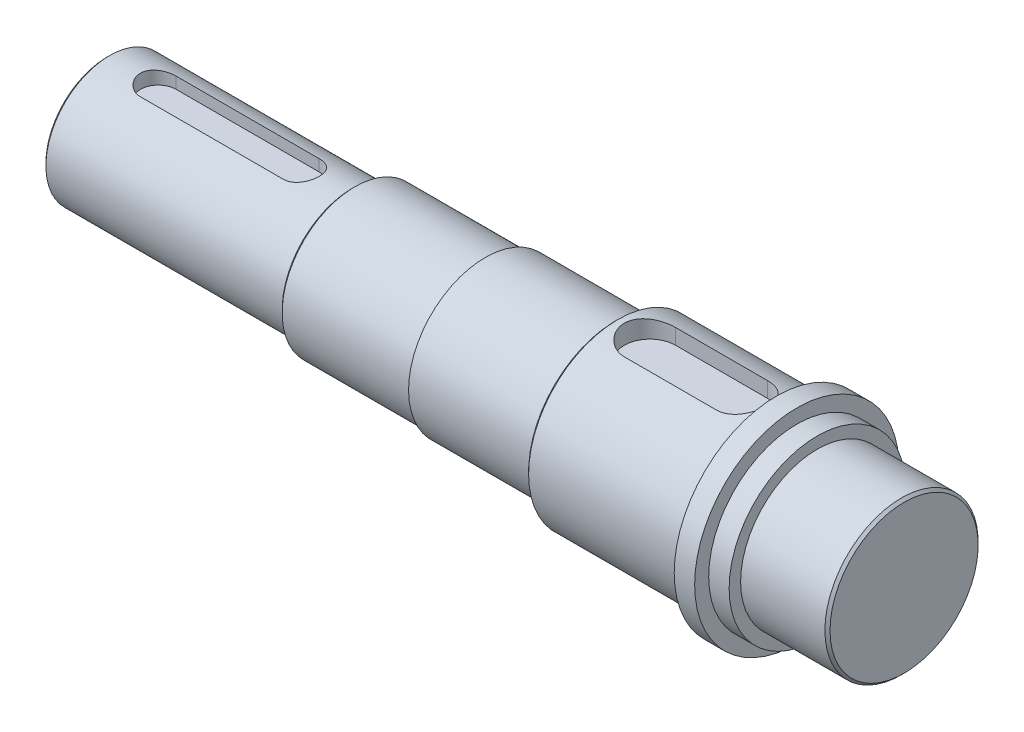
from build123d import *

# Parameters (mm, degrees)
CHAMFER1_SIZE      = 1
CHAMFER2_SIZE      = 1
FILLET1_R          = 0.5
CHAMFER3_SIZE      = 1
CHAMFER4_SIZE      = 1
FILLET2_R          = 0.5
CUT_EXTRUDE1_START = 19.5
CUT_EXTRUDE1_DEPTH = 20
CUT_EXTRUDE2_START = 27.5
CUT_EXTRUDE2_DEPTH = 20


with BuildPart() as part:
    # Sketch1 → Revolve3 (revolve)
    with BuildSketch(Plane.XY, mode=Mode.PRIVATE) as revolve3_sk:
        Polygon((0, 0), (0, 25), (96, 25), (96, 28.5), (148, 28.5), (148, 30), (199, 30), (199, 35), (262, 35), (262, 40), (270, 40), (270, 34.5), (278, 34.5), (278, 30), (312, 30), (312, 0), align=None)
    revolve(revolve3_sk.sketch.rotate(Axis((0, 0, 0), (1, 0, 0)), 90), axis=Axis((0, 0, 0), (1, 0, 0)))

    # Chamfer1
    chamfer1_edges = [part.edges().sort_by_distance(p)[0] for p in [
        (0, 0, -25),
    ]]
    chamfer(chamfer1_edges, length=CHAMFER1_SIZE)

    # Chamfer2
    chamfer2_edges = [part.edges().sort_by_distance(p)[0] for p in [
        (312, 0, -30),
    ]]
    chamfer(chamfer2_edges, length=CHAMFER2_SIZE)

    # Fillet1
    fillet1_edges = [part.edges().sort_by_distance(p)[0] for p in [
        (148, 0, -28.5),
        (96, 0, -25),
    ]]
    fillet(fillet1_edges, radius=FILLET1_R)

    # Chamfer3
    chamfer3_edges = [part.edges().sort_by_distance(p)[0] for p in [
        (199, 0, -35),
    ]]
    chamfer(chamfer3_edges, length=CHAMFER3_SIZE)

    # Chamfer4
    chamfer4_edges = [part.edges().sort_by_distance(p)[0] for p in [
        (96, 0, -28.5),
    ]]
    chamfer(chamfer4_edges, length=CHAMFER4_SIZE)

    # Fillet2
    fillet2_edges = [part.edges().sort_by_distance(p)[0] for p in [
        (199, 0, -30),
    ]]
    fillet(fillet2_edges, radius=FILLET2_R)

    # Sketch2 → Cut-Extrude1 (cut)
    with BuildSketch(Plane(origin=(0, 0, 0), x_dir=(1, 0, 0), z_dir=(0, 1, 0)).offset(CUT_EXTRUDE1_START)):
        with BuildLine():
            Line((20, 7), (76, 7))
            ThreePointArc((76, 7), (83, 0), (76, -7))
            Line((76, -7), (20, -7))
            ThreePointArc((20, -7), (13, 0), (20, 7))
        make_face()
    extrude(amount=CUT_EXTRUDE1_DEPTH, mode=Mode.SUBTRACT)

    # Sketch3 → Cut-Extrude2 (cut)
    with BuildSketch(Plane(origin=(0, 0, 0), x_dir=(1, 0, 0), z_dir=(0, 1, 0)).offset(CUT_EXTRUDE2_START)):
        with BuildLine():
            Line((212.5, 10), (248.5, 10))
            ThreePointArc((248.5, 10), (258.5, 0), (248.5, -10))
            Line((248.5, -10), (212.5, -10))
            ThreePointArc((212.5, -10), (202.5, 0), (212.5, 10))
        make_face()
    extrude(amount=CUT_EXTRUDE2_DEPTH, mode=Mode.SUBTRACT)


solid = part.part
